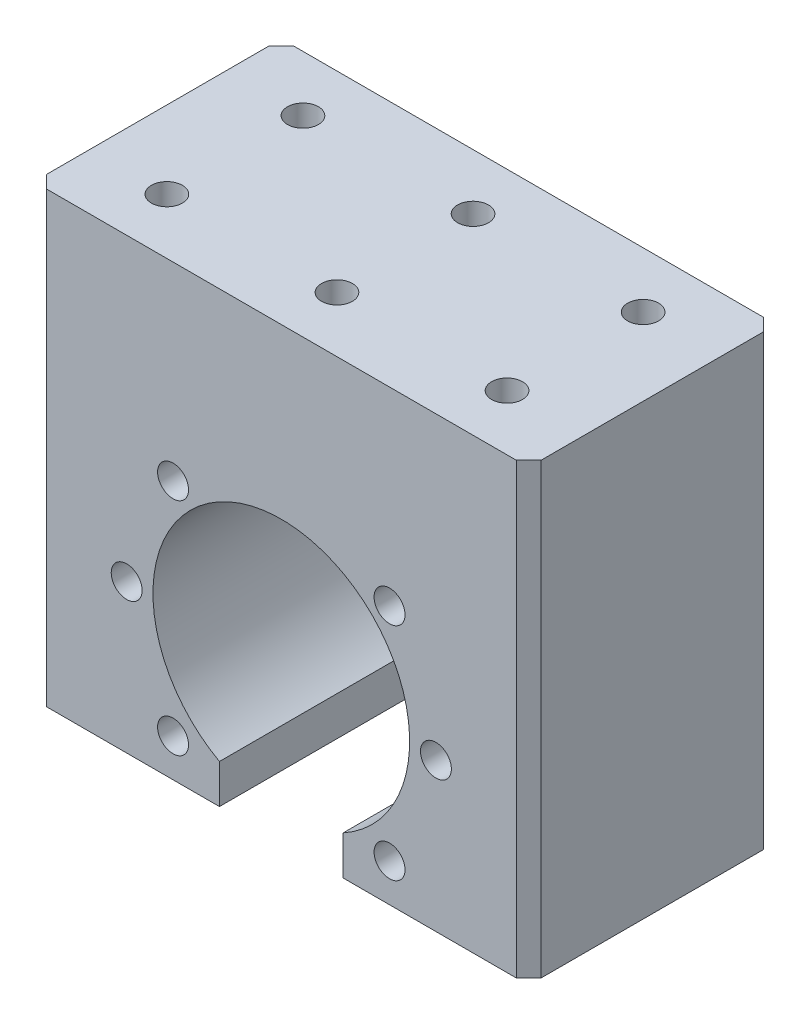
SolidWorks part; units mm, degrees
material "6061Al"
ref_plane "前视基准面" through (0, 0, 0) normal (0, 0, 1) x (1, 0, 0)
ref_plane "上视基准面" through (0, 0, 0) normal (0, 1, 0) x (1, 0, 0)
ref_plane "右视基准面" through (0, 0, 0) normal (1, 0, 0) x (0, 0, -1)
sketch "草图1" plane through (0, 0, 0) normal (0, 0, 1) x (1, 0, 0)
  line L1 (-40, -36.25) -> (40, -36.25)
  line L2 (-40, -36.25) -> (-40, 36.25)
  line L3 (-40, 36.25) -> (40, 36.25)
  line L4 (40, -36.25) -> (40, 36.25)
  line L5 (-40, -36.25) -> (40, 36.25) construction
  line L6 (-40, 36.25) -> (40, -36.25) construction
  circle A0 centre (0, -11.75) radius 20.75
  point P0 (0, 0)
  dimension "D4" = 41.5
  dimension "D1" = 80
  dimension "D2" = 72.5
  dimension "D3" = 24.5
extrude "凸台-拉伸1" add sketch "草图1" along normal mid plane 40
sketch "草图2" plane through (0, 0, 20) normal (0, 0, 1) x (1, 0, 0)
  line L0 (0, 0) -> (0, -36.25) construction
  line L1 (-40, -36.25) -> (40, -36.25) construction
  line L3 (-10, -29.9314) -> (10, -29.9314)
  line L4 (-10, -29.9314) -> (-10, -36.25)
  line L5 (-10, -36.25) -> (10, -36.25)
  line L6 (10, -29.9314) -> (10, -36.25)
  circle A0 centre (0, -11.75) radius 20.75 construction
  dimension "D1" = 20
extrude "切除-拉伸1" cut sketch "草图2" against normal through all
hole_wizard "M6 螺纹孔1" positions "草图3" profile "草图5" tap size "M6" standard "ISO" end condition through all
sketch "草图3" plane through (0, 0, -20) normal (0, 0, -1) x (-1, 0, 0)
  point P0 (-17.5, 5.6036)
  point P3 (17.5, 5.6036)
  point P6 (17.5, -30.1036)
  point P9 (-17.5, -30.1036)
  point P13 (-25, -12.25)
  point P16 (25, -12.25)
sketch "草图5" plane through (17.5, 5.6036, -20) normal (1, 0, 0) x (0, 1, 0)
  line L0 (0, 0) -> (0, 40)
  line L1 (0, 40) -> (2.5, 40)
  line L2 (2.5, 40) -> (2.5, 0)
  line L5 (2.5, 0) -> (0, 0)
  line L11 (0, -6.35) -> (0, 107.95) construction
  dimension "通孔螺纹孔钻头直径" = 5
  dimension "通孔螺纹孔钻头深度" = 40
cosmetic thread "孔螺蚊线1" parameters "D2"=6
cosmetic thread "孔螺蚊线2" parameters "D2"=6
cosmetic thread "孔螺蚊线3" parameters "D2"=6
cosmetic thread "孔螺蚊线4" parameters "D2"=6
cosmetic thread "孔螺蚊线11" parameters "D2"=6
cosmetic thread "孔螺蚊线12" parameters "D2"=6
hole_wizard "M6 螺纹孔2" positions "草图6" profile "草图7" tap size "M6" standard "ISO"
sketch "草图6" plane through (0, 36.25, 0) normal (0, 1, 0) x (1, 0, 0)
  line L0 (0, 0) -> (-40, 0) construction
  line L1 (-40, -20) -> (-40, 20) construction
  line L3 (0, 0) -> (0, 20) construction
  line L4 (40, 20) -> (-40, 20) construction
  point P0 (-27.5, 11)
  point P2 (-27.5, -11)
  point P19 (27.5, -11)
  point P20 (27.5, 11)
  point P21 (0, 11)
  point P23 (0, -11)
  dimension "D1" = 22
  dimension "D2" = 55
sketch "草图7" plane through (-27.5, 36.25, -11) normal (1, 0, 0) x (0, 0, 1)
  line L0 (0, 0) -> (0, 16.5022)
  line L1 (0, 16.5022) -> (2.5, 15)
  line L2 (2.5, 15) -> (2.5, 0)
  line L5 (2.5, 0) -> (0, 0)
  line L10 (0, 16.5022) -> (-2.5, 15) construction
  line L11 (0, -6.35) -> (0, 107.95) construction
  dimension "螺纹孔钻头直径" = 5
  dimension "螺纹孔钻头深度" = 15
  dimension "导头角度" = 118
cosmetic thread "孔螺蚊线5" parameters "D1"=12, "D2"=6
cosmetic thread "孔螺蚊线6" parameters "D1"=12, "D2"=6
cosmetic thread "孔螺蚊线7" parameters "D1"=12, "D2"=6
cosmetic thread "孔螺蚊线8" parameters "D1"=12, "D2"=6
cosmetic thread "孔螺蚊线9" parameters "D1"=12, "D2"=6
cosmetic thread "孔螺蚊线10" parameters "D1"=12, "D2"=6
chamfer "倒角1" distance 2 angle 45 4 edges at (40, 0, 20) (40, 0, -20) (-40, 0, -20) (-40, 0, 20)
